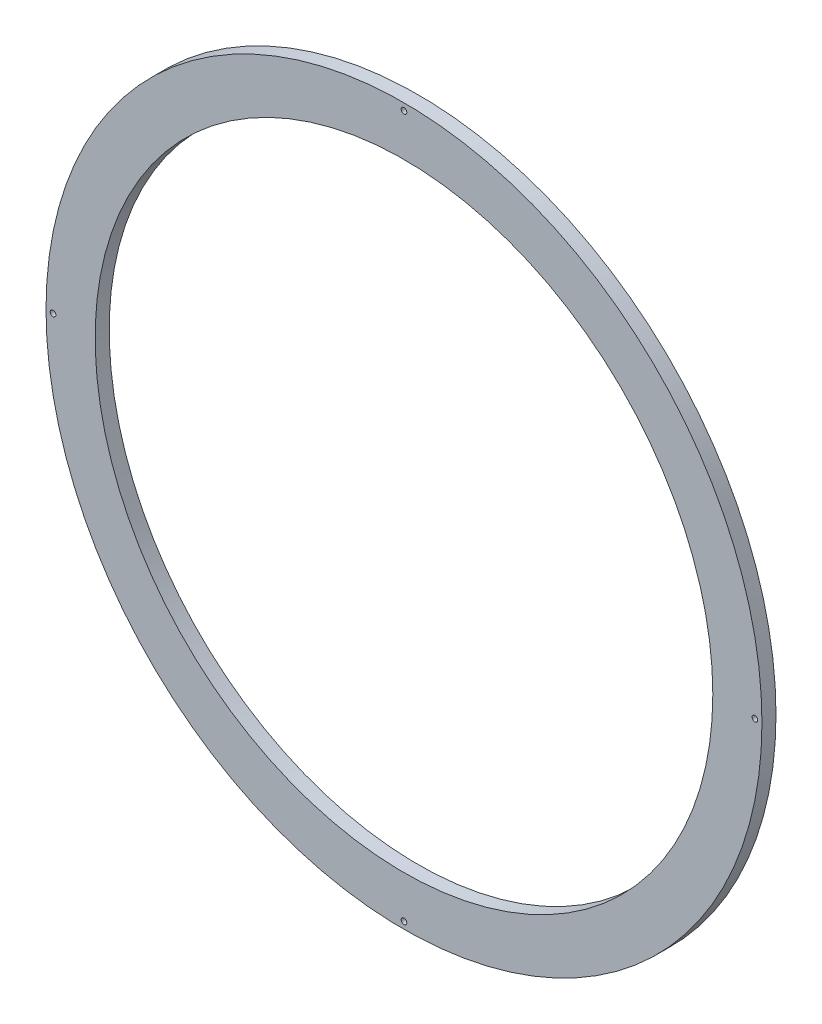
from build123d import *

# Parameters (mm, degrees)
SKETCH1_R           = 127.5
SKETCH1_R_2         = 110
BOSS_EXTRUDE1_DEPTH = 5
SKETCH4_R           = 1
CUT_EXTRUDE2_DEPTH  = 5
CIRPATTERN2_COUNT   = 4


with BuildPart() as part:
    # Sketch1 → Boss-Extrude1 (new body)
    with BuildSketch(Plane.XY):
        Circle(SKETCH1_R)
        Circle(SKETCH1_R_2, mode=Mode.SUBTRACT)
    extrude(amount=BOSS_EXTRUDE1_DEPTH)

    # Sketch4 → Cut-Extrude2 (cut)
    with BuildSketch(Plane.XY.offset(5)):
        with Locations((0, 125)):
            Circle(SKETCH4_R)
    cut_extrude2 = extrude(amount=-CUT_EXTRUDE2_DEPTH, mode=Mode.SUBTRACT)

    # CirPattern2: Cut-Extrude2 ×4 about axis
    cirpattern2_axis = Axis((0, 0, 0), (0, 0, 1))
    for i in range(1, CIRPATTERN2_COUNT):
        add(cut_extrude2.rotate(cirpattern2_axis, i * 360 / CIRPATTERN2_COUNT), mode=Mode.SUBTRACT)


solid = part.part
